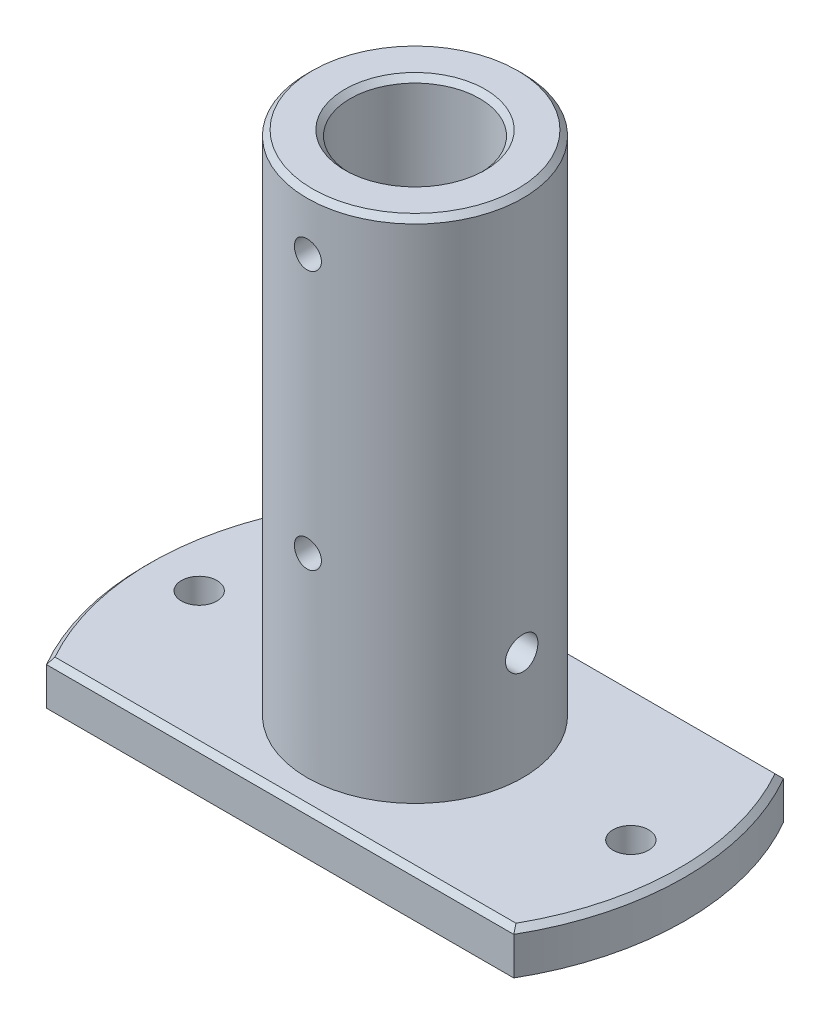
SolidWorks part; units mm, degrees
material "304"
ref_plane "Front Plane" through (0, 0, 0) normal (0, 0, 1) x (1, 0, 0)
ref_plane "Top Plane" through (0, 0, 0) normal (0, 1, 0) x (1, 0, 0)
ref_plane "Right Plane" through (0, 0, 0) normal (1, 0, 0) x (0, 0, -1)
sketch "Sketch1" plane through (0, 0, 0) normal (0, 0, 1) x (1, 0, 0)
  line L0 (0, 57.5825) -> (0, 0) construction
  line L1 (10, 51) -> (10, 4)
  line L2 (10, 4) -> (25, 4)
  line L3 (25, 4) -> (25, 0)
  line L4 (25, 0) -> (6, 0)
  line L5 (6, 0) -> (6, 51)
  line L6 (6, 51) -> (10, 51)
  dimension "D1" = 6
  dimension "D2" = 4
  dimension "D3" = 51
  dimension "D4" = 4
  dimension "D5" = 25
revolve "Revolve1" add sketch "Sketch1" angle 360 about L0
sketch "Sketch9" plane through (0, 4, 0) normal (0, 1, 0) x (1, 0, 0)
  line L1 (-26.1677, -12.5) -> (26.1677, -12.5)
  line L3 (-26.1677, 12.5) -> (26.1677, 12.5)
  arc A0 (-26.1677, -12.5) -> (26.1677, -12.5) centre (0, 0) ccw
  arc A1 (26.1677, 12.5) -> (-26.1677, 12.5) centre (0, 0) ccw
  circle A4 centre (0, 0) radius 10 construction
  circle A5 centre (0, 0) radius 6 construction
  dimension "D2" = 29
  dimension "D1" = 12.5
  dimension "D3" = 12.5
extrude "Cut-Extrude3" cut sketch "Sketch9" against normal blind 10
chamfer "Chamfer2" distance 0.5 angle 45 6 edges at (0, 51, 6) (0, 51, 10) (-25, 4, 0) (25, 4, 0) (0, 4, -12.5) (0, 4, 12.5)
ref_plane "Plane1" through (0, 0, 10) normal (0, 0, 1) x (1, 0, 0)
sketch "Sketch10" plane through (0, 0, 10) normal (0, 0, 1) x (1, 0, 0)
  line L0 (0, 0) -> (0, 51) construction
  line L1 (6.5, 51) -> (-6.5, 51) construction
  line L2 (9.5, 51) -> (-9.5, 51) construction
  point P5 (0, 46)
  point P6 (0, 22)
  dimension "D1" = 24
  dimension "D2" = 5
hole_wizard "M3 Tapped Hole1" positions "3DSketch1" profile "Sketch11" tap size "M3" standard "GB"
sketch3d "3DSketch1"
  point P7 (0, 22, 10)
  point P9 (0, 46, 10)
sketch "Sketch11" plane through (0, 22, 10) normal (1, 0, 0) x (0, -1, 0)
  line L0 (0, 0) -> (0, 9.2511)
  line L1 (0, 9.2511) -> (1.25, 8.5)
  line L2 (1.25, 8.5) -> (1.25, 0)
  line L5 (1.25, 0) -> (0, 0)
  line L10 (0, 9.2511) -> (-1.25, 8.5) construction
  line L11 (0, -6.35) -> (0, 107.95) construction
  dimension "螺纹孔钻头直径" = 2.5
  dimension "螺纹孔钻头深度" = 8.5
  dimension "导头角度" = 118
cosmetic thread "Cosmetic Thread3" parameters "D1"=4.1317, "D2"=3
cosmetic thread "Cosmetic Thread4" parameters "D1"=4.1317, "D2"=3
sketch "Sketch14" plane through (0, 0, 0) normal (0, -1, 0) x (1, 0, 0)
  circle A0 centre (0, 0) radius 6 construction
  point P0 (-20, 0)
  point P1 (20, 0)
  dimension "D1" = 20
  dimension "D2" = 20
hole_wizard "M4 Tapped Hole1" positions "3DSketch3" profile "Sketch15" tap size "M4" standard "GB"
sketch3d "3DSketch3"
  point P0 (-20, 0, 0)
  point P3 (20, 0, 0)
sketch "Sketch15" plane through (-20, 0, 0) normal (1, 0, 0) x (0, 0, -1)
  line L0 (0, 0) -> (0, 12.4914)
  line L1 (0, 12.4914) -> (1.65, 11.5)
  line L2 (1.65, 11.5) -> (1.65, 0)
  line L5 (1.65, 0) -> (0, 0)
  line L10 (0, 12.4914) -> (-1.65, 11.5) construction
  line L11 (0, -6.35) -> (0, 107.95) construction
  dimension "螺纹孔钻头直径" = 3.3
  dimension "螺纹孔钻头深度" = 11.5
  dimension "导头角度" = 118
cosmetic thread "Cosmetic Thread5" parameters "D1"=4, "D2"=4
cosmetic thread "Cosmetic Thread6" parameters "D1"=4, "D2"=4
sketch "Sketch16" plane through (0, 0, 0) normal (1, 0, 0) x (0, 0, -1)
  line L2 (-12.5, 0) -> (12.5, 0) construction
  circle A0 centre (0, 14) radius 1.5
  dimension "D1" = 3
  dimension "D2" = 14
extrude "Cut-Extrude4" cut sketch "Sketch16" against normal mid plane 53
